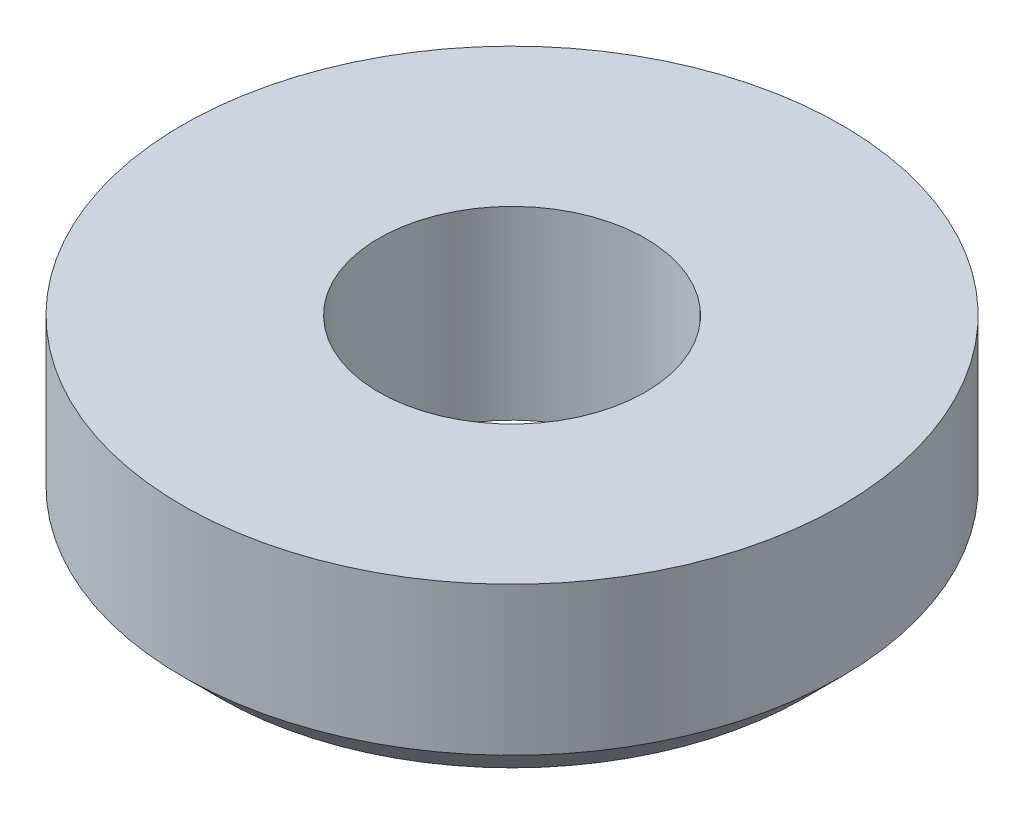
from build123d import *

# Parameters (mm, degrees)
SKETCH1_W     = 26.5
SKETCH1_H     = 25
CHAMFER1_SIZE = 5


with BuildPart() as part:
    # Sketch1 → Revolve1 (revolve)
    with BuildSketch(Plane.XY):
        with Locations((31.25, 12.5)):
            Rectangle(SKETCH1_W, SKETCH1_H)
    revolve(axis=Axis((0, -964.354117897, 0), (0, 1, 0)))

    # Chamfer1
    chamfer1_edges = [part.edges().sort_by_distance(p)[0] for p in [
        (-44.5, 0, 0),
    ]]
    chamfer(chamfer1_edges, length=CHAMFER1_SIZE)


solid = part.part
